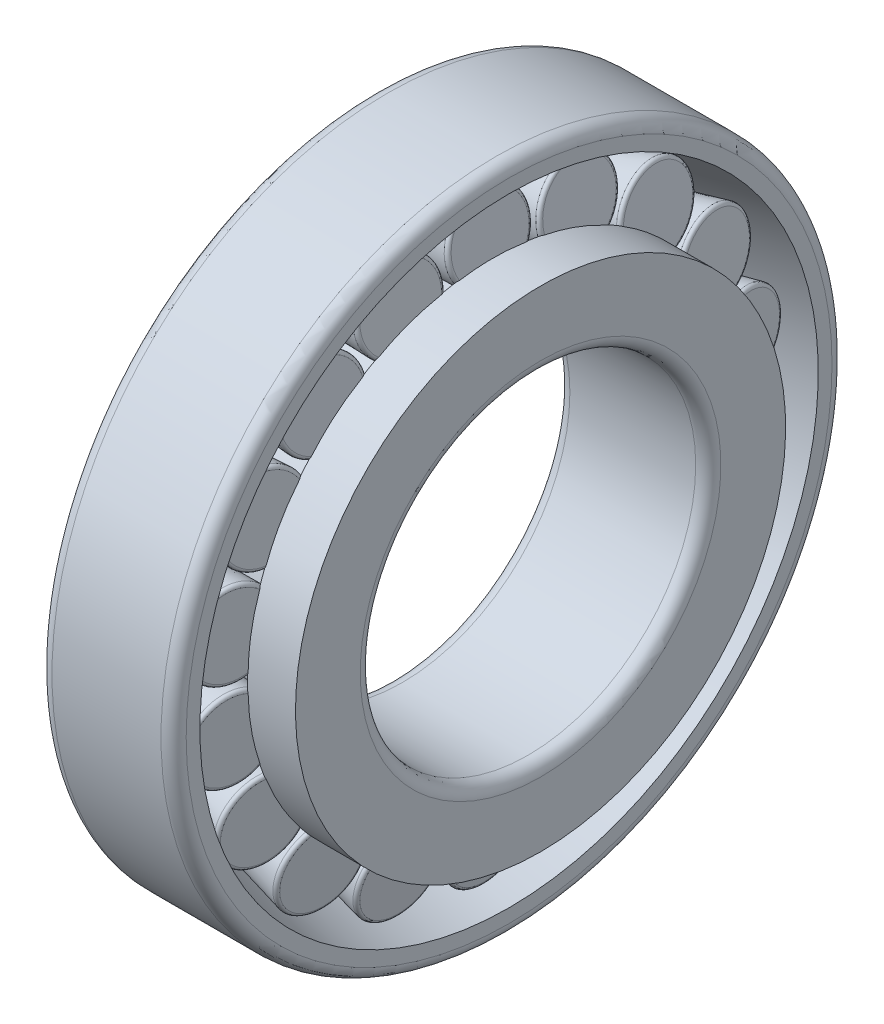
from build123d import *

# Parameters (mm, degrees)
CIRCULAR_PATTERN1_COUNT = 18


with BuildPart() as part:
    # Sketch1 → Revolve1 (revolve)
    with BuildSketch(Plane.XY, mode=Mode.PRIVATE) as revolve1_sk:
        with BuildLine():
            Line((11.75, 29.221405533), (6.022914246, 29.221405533))
            Line((6.022914246, 29.221405533), (6.5, 26.221405533))
            Line((6.5, 26.221405533), (-3.979556599, 25.481986561))
            Line((-3.979556599, 25.481986561), (-4.218099476, 26.981986561))
            Line((-4.218099476, 26.981986561), (-6.25, 26.981986561))
            Line((-6.25, 26.981986561), (-6.25, 21.5))
            ThreePointArc((-6.25, 21.5), (-5.810660172, 20.439339828), (-4.75, 20))
            Line((-4.75, 20), (10.25, 20))
            ThreePointArc((10.25, 20), (11.310660172, 20.439339828), (11.75, 21.5))
            Line((11.75, 21.5), (11.75, 29.221405533))
        make_face()
    revolve(revolve1_sk.sketch.rotate(Axis((11.75, 0, 0), (1, 0, 0)), 180), axis=Axis((11.75, 0, 0), (1, 0, 0)))

    # Sketch2 → Revolve2 (revolve)
    with BuildSketch(Plane.XY, mode=Mode.PRIVATE) as revolve2_sk:
        with BuildLine():
            Line((-4.640780097, 29.512533501), (5.734476712, 31.162495908))
            Line((5.734476712, 31.162495908), (6.454621517, 26.634097411))
            ThreePointArc((6.454621517, 26.634097411), (6.37278523, 26.322466289), (6.087738874, 26.172267394))
            Line((6.087738874, 26.172267394), (-3.63080663, 25.486544019))
            ThreePointArc((-3.63080663, 25.486544019), (-3.907769044, 25.572352373), (-4.053995871, 25.822730022))
            Line((-4.053995871, 25.822730022), (-4.640780097, 29.512533501))
        make_face()
    revolve2 = revolve(revolve2_sk.sketch.rotate(Axis((-4.640780097, 29.512533501, 0), (0.9875898549665195, 0.15705501700744515, 0)), 4.715305364), axis=Axis((-4.640780097, 29.512533501, 0), (0.9875898549665195, 0.15705501700744515, 0)))

    # Sketch3 → Revolve3 (revolve)
    with BuildSketch(Plane.XY, mode=Mode.PRIVATE) as revolve3_sk:
        with BuildLine():
            Line((-8, 32.865), (8, 36.864927762))
            Line((8, 36.864927762), (8, 38.5))
            ThreePointArc((8, 38.5), (7.560660172, 39.560660172), (6.5, 40))
            Line((6.5, 40), (-6.5, 40))
            ThreePointArc((-6.5, 40), (-7.560660172, 39.560660172), (-8, 38.5))
            Line((-8, 38.5), (-8, 32.865))
        make_face()
    revolve(revolve3_sk.sketch.rotate(Axis((11.75, 0, 0), (1, 0, 0)), 180), axis=Axis((11.75, 0, 0), (1, 0, 0)))

    # Circular-Pattern1: Revolve2 ×18 about axis
    circular_pattern1_axis = Axis((0, 0, 0), (1, 0, 0))
    for i in range(1, CIRCULAR_PATTERN1_COUNT):
        add(revolve2.rotate(circular_pattern1_axis, i * 360 / CIRCULAR_PATTERN1_COUNT))


solid = part.part
